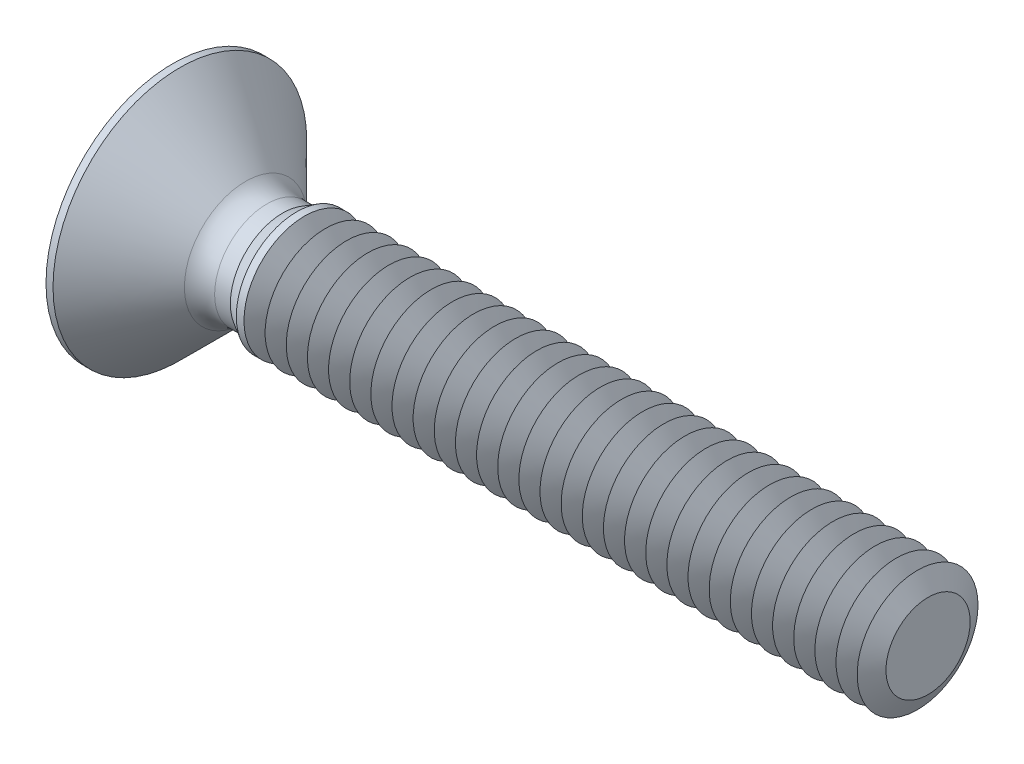
SolidWorks part; units mm, degrees
revolve "基体-旋转" add sketch "草图1" angle 360 about L0
sketch "草图1" plane through (0, 0, 0) normal (0, 0, 1) x (1, 0, 0)
  line L0 (0, 0) -> (4.4175, 0) construction
  line L1 (0, 0) -> (0, 4.2)
  line L2 (0, 4.2) -> (0.232, 4.2)
  line L3 (0.232, 4.2) -> (2.4071, 2.0249)
  line L4 (3.1142, 1.732) -> (3.6358, 1.732)
  line L5 (3.6358, 1.732) -> (4.1, 2)
  line L6 (4.1, 2) -> (25, 2)
  line L7 (25, 2) -> (25, 0)
  line L8 (0, 0) -> (25, 0)
  arc A0 (3.1142, 1.732) -> (2.4071, 2.0249) centre (3.1142, 2.732) cw
  point P12 (2.7, 1.732)
cosmetic thread "装饰螺纹线2" parameters "D1"=20.9, "D2"=3.3
material "4.8级"
ref_plane "前视" through (0, 0, 0) normal (0, 0, 1) x (1, 0, 0)
ref_plane "上视" through (0, 0, 0) normal (0, 1, 0) x (1, 0, 0)
ref_plane "右视" through (0, 0, 0) normal (1, 0, 0) x (0, 0, -1)
sketch "尺寸草图" plane through (0, 0, 0) normal (0, 0, 1) x (1, 0, 0)
  line L0 (0, 0) -> (25, 0)
  point P3 (2.7, 0)
  point P4 (1.4, 0)
  point P5 (4, 0)
  point P6 (8.4, 0)
  point P7 (20.4, 0)
  point P8 (3.5943, 0)
  point P9 (24, 0)
  point P10 (22.4, 0)
  point P11 (24.3, 0)
sketch "草图2" plane through (0, 0, 0) normal (0, 0, 1) x (1, 0, 0)
  line L0 (24.6538, 2) -> (25.3538, 2)
  line L1 (25.3538, 2) -> (25, 1.3938)
  line L2 (25, 1.3938) -> (24.6538, 2)
  line L3 (25, -2) -> (25, 2) construction
  line L6 (0, 0) -> (-0.4315, 0) construction
revolve "切除-旋转1" cut sketch "草图2" angle 360 about L6
pattern_linear "阵列(线性)1" count 30 spacing 0.7 along (-1, 0, 0) of "切除-旋转1"
sketch "草图3" plane through (0, 0, 0) normal (-1, 0, 0) x (0, 0, 1)
  line L0 (0, 0) -> (1.6329, 0) construction
  line L1 (0, 0) -> (0, 0.8499) construction
  line L2 (-2.3, 0.35) -> (2.3, 0.35)
  line L3 (-2.3, 0.35) -> (-2.3, -0.35)
  line L4 (-2.3, -0.35) -> (2.3, -0.35)
  line L5 (2.3, 0.35) -> (2.3, -0.35)
ref_plane "基准面1" through (2.6, 0, 0) normal (-1, 0, 0) x (0, 0, 1)
sketch "草图4" plane through (2.6, 0, 0) normal (-1, 0, 0) x (0, 0, 1)
  point P0 (0, 0)
loft "切除-放样1" cut profiles "草图3", "草图4"
pattern_circular "阵列(圆周)1" count 2 every 90 about axis through (0, 0, 0) along (1, 0, 0) of "切除-放样1"
equation "\"l@草图1\" = \"l@尺寸草图\""
equation "\"k@草图1\" = \"k@尺寸草图\""
equation "\"a@草图1\" = \"a@尺寸草图\""
equation "\"d@草图1\" = \"d@尺寸草图\""
equation "\"dk@草图1\" = \"dk@尺寸草图\""
equation "\"D2@草图1\" = \"r@尺寸草图\""
equation "\"m@草图3\" = \"m@尺寸草图\""
equation "\"h@基准面1\" = \"h@尺寸草图\""
equation "\"D3@阵列(线性)1\" = \"p@尺寸草图\""
equation "\"D3@草图2\" = \"d@草图1\" / 2"
equation "\"D1@装饰螺纹线2\" = \"l@草图1\" - \"k@草图1\" - \"a@草图1\""
equation "\"D2@装饰螺纹线2\" = \"d@尺寸草图\"- \"p@尺寸草图\""
equation "\"D1@阵列(线性)1\" = (  \"l@草图1\" - \"k@草图1\" - \"a@草图1\" )  / \"p@尺寸草图\""
equation "\"D1@草图3\" = \"p@尺寸草图\""
equation "\"D1@草图1\" = \"d@尺寸草图\"*0.866"
equation "\"D2@草图2\" = \"p@尺寸草图\"*0.866"
equation "\"D1@草图2\" = \"p@尺寸草图\""
